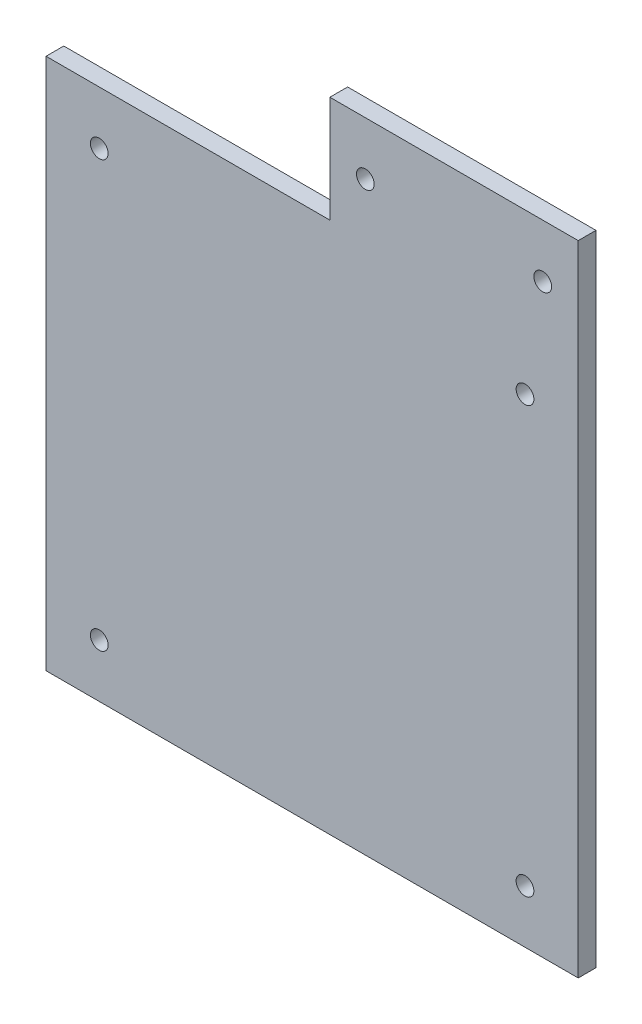
SolidWorks part; units mm, degrees
ref_plane "前视基准面" through (0, 0, 0) normal (0, 0, 1) x (1, 0, 0)
ref_plane "上视基准面" through (0, 0, 0) normal (0, 1, 0) x (1, 0, 0)
ref_plane "右视基准面" through (0, 0, 0) normal (1, 0, 0) x (0, 0, -1)
sketch "草图1" plane through (0, 0, 0) normal (0, 0, 1) x (1, 0, 0)
  line L0 (0, 0) -> (300, 0)
  line L1 (300, 0) -> (300, 300)
  line L2 (200, 300) -> (0, 300)
  line L3 (0, 300) -> (0, 0)
  line L4 (300, 300) -> (300, 360)
  line L5 (300, 360) -> (200, 360)
  line L6 (200, 360) -> (200, 300)
  line L7 (0, 0) -> (30, 0)
  circle A0 centre (30, 30) radius 5
  circle A1 centre (270, 30) radius 5
  circle A2 centre (270, 270) radius 5
  circle A3 centre (30, 270) radius 5
extrude "凸台-拉伸1" add sketch "草图1" along normal blind 10 contours L5 L6 L2 L3 L0 L1 L4 A1 A0 A2 A3
sketch "草图3" plane through (200, 0, 0) normal (-1, 0, 0) x (0, 0, 1)
  line L8 (0, 360) -> (0, 300)
  line L9 (0, 300) -> (10, 300)
  line L10 (10, 300) -> (10, 360)
  line L11 (10, 360) -> (0, 360)
  line L12 (0, 360) -> (0, 300)
  line L13 (0, 300) -> (10, 300)
  line L14 (10, 300) -> (10, 360)
  line L15 (10, 360) -> (0, 360)
  dimension "D1" = 0
extrude "凸台-拉伸2" add sketch "草图3" along normal blind 40
sketch "草图4" plane through (0, 0, 10) normal (0, 0, 1) x (1, 0, 0)
  line L0 (160, 330) -> (300, 330)
  line L1 (160, 300) -> (160, 360) construction
  line L2 (300, 0) -> (300, 360) construction
  line L3 (300, 330) -> (280, 330)
  line L4 (230, 330) -> (230, 343.5644)
  circle A0 centre (280, 330) radius 5
  circle A1 centre (180, 330) radius 5
extrude "切除-拉伸2" cut sketch "草图4" against normal blind 40 contours A1 L0 | A1 L0 | L0 A0 | L0 A0
